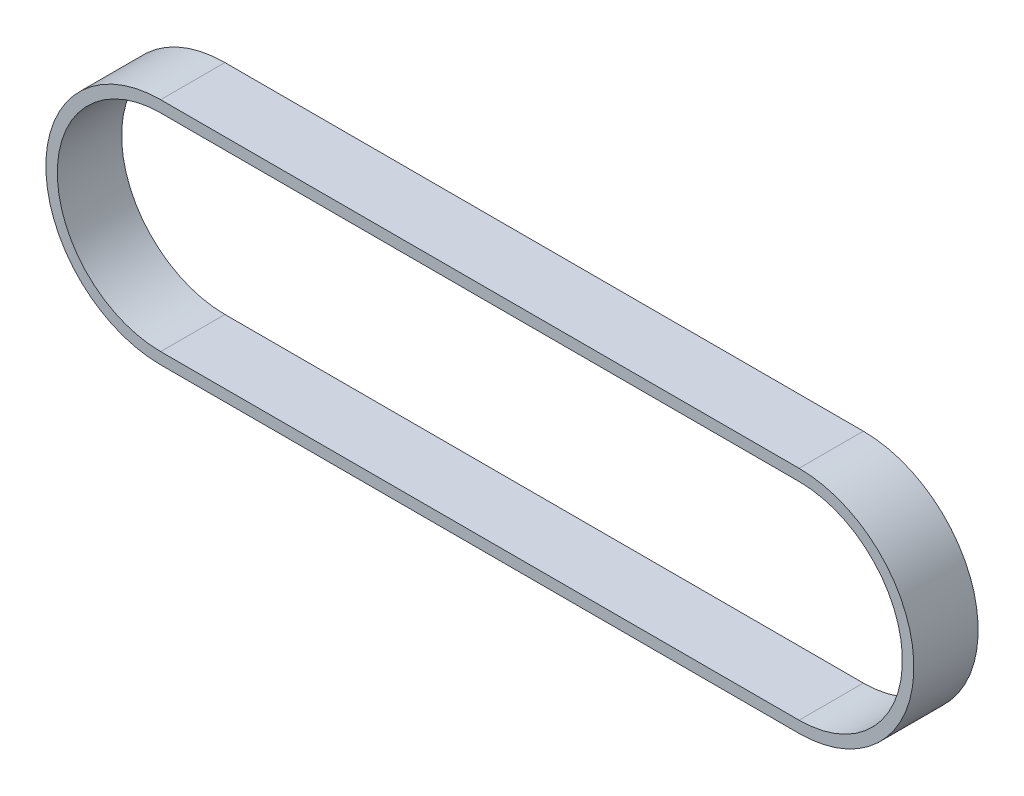
SolidWorks part; units mm, degrees
ref_plane "前视基准面" through (0, 0, 0) normal (0, 0, 1) x (1, 0, 0)
ref_plane "上视基准面" through (0, 0, 0) normal (0, 1, 0) x (1, 0, 0)
ref_plane "右视基准面" through (0, 0, 0) normal (1, 0, 0) x (0, 0, -1)
sketch "草图1" plane through (0, 0, 0) normal (0, 0, 1) x (1, 0, 0)
  line L0 (0, 0) -> (278, 0) construction
  line L1 (0, 45) -> (278, 45)
  line L2 (0, -45) -> (278, -45)
  line L3 (0, 50) -> (278, 50)
  line L4 (0, -50) -> (278, -50)
  arc A0 (0, 45) -> (0, -45) centre (0, 0) ccw
  arc A1 (278, -45) -> (278, 45) centre (278, 0) ccw
  arc A2 (278, -50) -> (278, 50) centre (278, 0) ccw
  arc A3 (0, 50) -> (0, -50) centre (0, 0) ccw
  point P3 (139, 0)
  dimension "D1" = 278
  dimension "D2" = 90
  dimension "D3" = 5
extrude "凸台-拉伸1" add sketch "草图1" along normal blind 28
